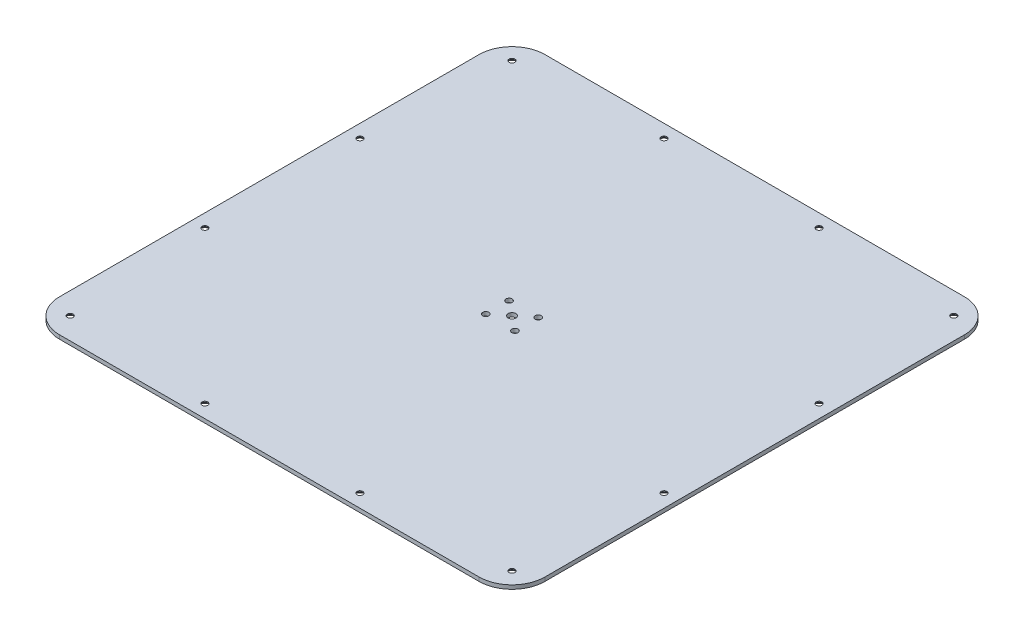
from build123d import *

# Parameters (mm, degrees)
EXTRUDE_1_DEPTH          = 1
EXTRUDE_1_DEPTH_BACK     = 1
CUT_EXTRUDE_1_DEPTH      = 178.133071446
CUT_EXTRUDE_1_DEPTH_BACK = 178.133071446
SKETCH_2_R               = 1.5
SKETCH_2_R_2             = 1.6
SKETCH_2_R_3             = 2
SKETCH_3_R               = 3
EXTRUDE_2_DEPTH          = 7.5
HOLE_WIZARD_M4_1_D       = 3.3
HOLE_WIZARD_M4_1_DEPTH   = 7
HOLE_WIZARD_M4_1_TIP     = 0.952627944
CHAMFER_1_SIZE           = 1.5
SKETCH_7_R               = 1.25
EXTRUDE_3_DEPTH          = 15
CHAMFER_2_SIZE           = 0.2


with BuildPart() as part:
    # 草图1 → 凸台-拉伸1 (new, two sides: drawn at the far end of the back side and taken through both)
    with BuildSketch(Plane(origin=(0, 0, 0), x_dir=(1, 0, 0), z_dir=(0, 1, 0)).offset(-EXTRUDE_1_DEPTH_BACK)):
        with BuildLine():
            Line((-108.25, -125.25), (108.25, -125.25))
            ThreePointArc((108.25, -125.25), (120.27081528, -120.27081528), (125.25, -108.25))
            Line((125.25, -108.25), (125.25, 108.25))
            ThreePointArc((125.25, 108.25), (120.27081528, 120.27081528), (108.25, 125.25))
            Line((108.25, 125.25), (-108.25, 125.25))
            ThreePointArc((-108.25, 125.25), (-120.27081528, 120.27081528), (-125.25, 108.25))
            Line((-125.25, 108.25), (-125.25, -108.25))
            ThreePointArc((-125.25, -108.25), (-120.27081528, -120.27081528), (-108.25, -125.25))
        make_face()
    extrude(amount=EXTRUDE_1_DEPTH + EXTRUDE_1_DEPTH_BACK)

    # 草图2 → 切除-拉伸1 (cut, two sides: drawn at the far end of the back side and taken through both)
    with BuildSketch(Plane(origin=(0, 0, 0), x_dir=(1, 0, 0), z_dir=(0, 1, 0)).offset(-CUT_EXTRUDE_1_DEPTH_BACK)):
        with Locations(Location((-114, -114, 0), (0, 0, 270))):
            Circle(SKETCH_2_R)
        with Locations(Location((-40, -118.5, 0), (0, 0, 270))):
            Circle(SKETCH_2_R)
        with Locations(Location((40, -118.5, 0), (0, 0, 270))):
            Circle(SKETCH_2_R)
        with Locations(Location((-114, 114, 0), (0, 0, 270))):
            Circle(SKETCH_2_R)
        with Locations(Location((-118.5, 40, 0), (0, 0, 270))):
            Circle(SKETCH_2_R)
        with Locations(Location((-118.5, -40, 0), (0, 0, 270))):
            Circle(SKETCH_2_R)
        with Locations(Location((114, 114, 0), (0, 0, 270))):
            Circle(SKETCH_2_R)
        with Locations(Location((40, 118.5, 0), (0, 0, 270))):
            Circle(SKETCH_2_R)
        with Locations(Location((-40, 118.5, 0), (0, 0, 270))):
            Circle(SKETCH_2_R)
        with Locations(Location((114, -114, 0), (0, 0, 270))):
            Circle(SKETCH_2_R)
        with Locations(Location((118.5, -40, 0), (0, 0, 270))):
            Circle(SKETCH_2_R)
        with Locations(Location((118.5, 40, 0), (0, 0, 270))):
            Circle(SKETCH_2_R)
        with Locations(Location((-7.5, -6, 0), (0, 0, 270))):
            Circle(SKETCH_2_R_2)
        with Locations(Location((7.5, -6, 0), (0, 0, 270))):
            Circle(SKETCH_2_R_2)
        with Locations(Location((7.5, 6, 0), (0, 0, 270))):
            Circle(SKETCH_2_R_2)
        with Locations(Location((-7.5, 6, 0), (0, 0, 270))):
            Circle(SKETCH_2_R_2)
        with Locations(Location((0, 0, 0), (0, 0, 270))):
            Circle(SKETCH_2_R_3)
    extrude(amount=CUT_EXTRUDE_1_DEPTH + CUT_EXTRUDE_1_DEPTH_BACK, mode=Mode.SUBTRACT)

    # 草图3 → 凸台-拉伸2 (add)
    with BuildSketch(Plane.XZ.offset(1)):
        with Locations(Location((-102.045584412, -102.045584412, 0), (0, 0, 270))):
            Circle(SKETCH_3_R)
        with Locations(Location((-55, -104.35, 0), (0, 0, 270))):
            Circle(SKETCH_3_R)
        with Locations(Location((0, -104.35, 0), (0, 0, 270))):
            Circle(SKETCH_3_R)
        with Locations(Location((55, -104.35, 0), (0, 0, 270))):
            Circle(SKETCH_3_R)
        with Locations(Location((102.045584412, -102.045584412, 0), (0, 0, 270))):
            Circle(SKETCH_3_R)
        with Locations(Location((104.35, -55, 0), (0, 0, 270))):
            Circle(SKETCH_3_R)
        with Locations(Location((105, 0, 0), (0, 0, 270))):
            Circle(SKETCH_3_R)
        with Locations(Location((104.35, 55, 0), (0, 0, 270))):
            Circle(SKETCH_3_R)
        with Locations(Location((102.045584412, 102.045584412, 0), (0, 0, 270))):
            Circle(SKETCH_3_R)
        with Locations(Location((55, 104.35, 0), (0, 0, 270))):
            Circle(SKETCH_3_R)
        with Locations(Location((0, 104.35, 0), (0, 0, 270))):
            Circle(SKETCH_3_R)
        with Locations(Location((-55, 104.35, 0), (0, 0, 270))):
            Circle(SKETCH_3_R)
        with Locations(Location((-102.045584412, 102.045584412, 0), (0, 0, 270))):
            Circle(SKETCH_3_R)
        with Locations(Location((-104.35, 34.045584412, 0), (0, 0, 270))):
            Circle(SKETCH_3_R)
        with Locations(Location((-104.35, -34.045584412, 0), (0, 0, 270))):
            Circle(SKETCH_3_R)
    extrude(amount=EXTRUDE_2_DEPTH)

    # M4 螺纹孔1
    with Locations(Plane(origin=(0, -8.5, 0), x_dir=(-1, 0, 0), z_dir=(0, -1, 0))):
        with Locations((102.045584412, -102.045584412), (55, -104.35), (0, -104.35), (-55, -104.35), (-102.045584412, -102.045584412), (-104.35, -55), (-105, 0), (-104.35, 55), (-102.045584412, 102.045584412), (-55, 104.35), (0, 104.35), (55, 104.35), (102.045584412, 102.045584412), (104.35, 34.045584412), (104.35, -34.045584412)):
            Hole(HOLE_WIZARD_M4_1_D / 2, depth=HOLE_WIZARD_M4_1_DEPTH)
            with Locations((0, 0, -(HOLE_WIZARD_M4_1_DEPTH + HOLE_WIZARD_M4_1_TIP / 2))):  # 120° drill point
                Cone(0, HOLE_WIZARD_M4_1_D / 2, HOLE_WIZARD_M4_1_TIP, mode=Mode.SUBTRACT)

    # 倒角1
    chamfer_1_edges = [part.edges().sort_by_distance(p)[0] for p in [
        (-114, -1, 112.5),
        (-40, -1, 117),
        (40, -1, 117),
        (-114, -1, -115.5),
        (-118.5, -1, -41.5),
        (-118.5, -1, 38.5),
        (114, -1, -115.5),
        (40, -1, -120),
        (-40, -1, -120),
        (114, -1, 112.5),
        (118.5, -1, 38.5),
        (118.5, -1, -41.5),
    ]]
    chamfer(chamfer_1_edges, length=CHAMFER_1_SIZE)

    # 草图7 → 凸台-拉伸3 (add)
    with BuildSketch(Plane(origin=(0, -1, 0), x_dir=(-1, 0, 0), z_dir=(0, -1, 0))):
        with Locations(Location((4.55, 15.75, 0), (0, 0, 90))):
            Circle(SKETCH_7_R)
        with Locations(Location((-72.45, 15.75, 0), (0, 0, 90))):
            Circle(SKETCH_7_R)
        with Locations(Location((-72.45, -90.25, 0), (0, 0, 90))):
            Circle(SKETCH_7_R)
        with Locations(Location((4.55, -90.25, 0), (0, 0, 90))):
            Circle(SKETCH_7_R)
        with Locations(Location((-51.9, 11.85, 0), (0, 0, 90))):
            Circle(SKETCH_7_R)
        with Locations(Location((-40.7, 11.85, 0), (0, 0, 90))):
            Circle(SKETCH_7_R)
        with Locations(Location((-89.1, -78.125, 0), (0, 0, 90))):
            Circle(SKETCH_7_R)
        with Locations(Location((-89.1, -66.325, 0), (0, 0, 90))):
            Circle(SKETCH_7_R)
    extrude(amount=EXTRUDE_3_DEPTH)

    # 倒角2
    chamfer_2_edges = [part.edges().sort_by_distance(p)[0] for p in [
        (-4.55, -16, -14.5),
        (72.45, -16, -14.5),
        (72.45, -16, 91.5),
        (-4.55, -16, 91.5),
        (51.9, -16, -10.6),
        (40.7, -16, -10.6),
        (89.1, -16, 79.375),
        (89.1, -16, 67.575),
    ]]
    chamfer(chamfer_2_edges, length=CHAMFER_2_SIZE)


solid = part.part
